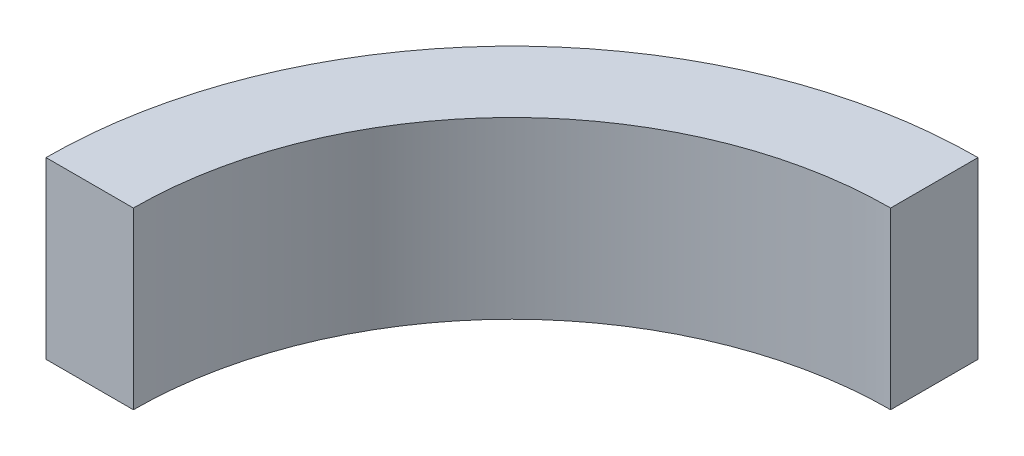
from build123d import *

# Parameters (mm, degrees)
EXTRUDE_1_DEPTH = 30


with BuildPart() as part:
    # 草图1 → 凸台-拉伸1 (new body)
    with BuildSketch(Plane(origin=(0, 0, 0), x_dir=(1, 0, 0), z_dir=(0, 1, 0))):
        with BuildLine():
            Line((-80, 0), (-65, 0))
            ThreePointArc((-65, 0), (-45.961940777, 45.961940777), (0, 65))
            Line((0, 65), (0, 80))
            ThreePointArc((0, 80), (-56.568542495, 56.568542495), (-80, 0))
        make_face()
    extrude(amount=EXTRUDE_1_DEPTH)


solid = part.part
